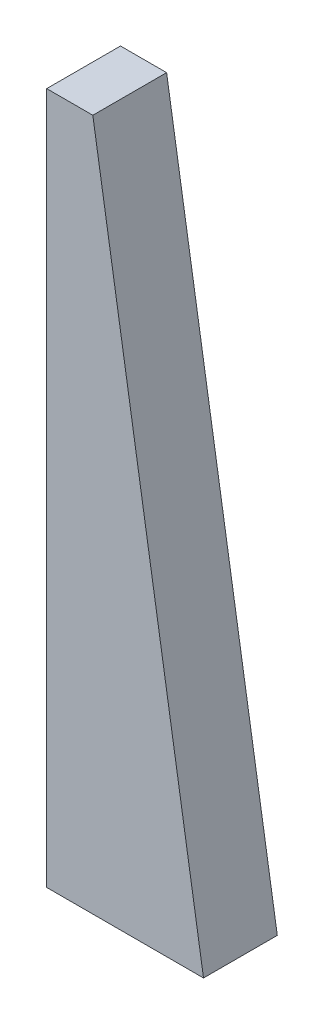
from build123d import *

# Parameters (mm, degrees)
EXTRUDE1_DEPTH = 8


with BuildPart() as part:
    # Sketch1 → Extrude1 (new, symmetric)
    with BuildSketch(Plane.XY):
        Polygon((0, 0), (34, 0), (10, 150), (0, 150), align=None)
    extrude(amount=EXTRUDE1_DEPTH, both=True)


solid = part.part
